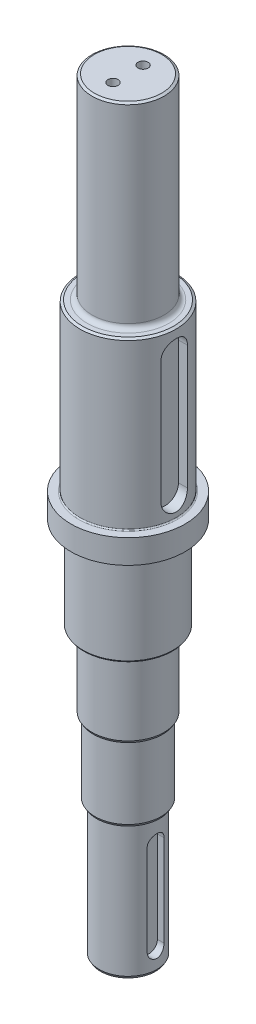
SolidWorks part; units mm, degrees
ref_plane "Front Plane" through (0, 0, 0) normal (0, 0, 1) x (1, 0, 0)
ref_plane "Top Plane" through (0, 0, 0) normal (0, 1, 0) x (1, 0, 0)
ref_plane "Right Plane" through (0, 0, 0) normal (1, 0, 0) x (0, 0, -1)
sketch "Sketch2" plane through (0, 0, 0) normal (0, 0, 1) x (1, 0, 0)
  line L0 (0, -318) -> (0, 318)
  line L1 (0, 318) -> (30, 318)
  line L2 (30, 318) -> (30, 155)
  line L3 (30, 155) -> (40, 155)
  line L4 (40, 155) -> (40, 17)
  line L5 (40, 17) -> (47.5, 17)
  line L6 (47.5, 17) -> (47.5, -3)
  line L7 (47.5, -3) -> (37.5, -3)
  line L8 (37.5, -3) -> (37.5, -80)
  line L9 (37.5, -80) -> (30, -80)
  line L10 (30, -80) -> (30, -144)
  line L11 (30, -144) -> (27.5, -144)
  line L12 (27.5, -144) -> (27.5, -206)
  line L13 (27.5, -206) -> (24, -206)
  line L14 (24, -206) -> (24, -318)
  line L17 (24, -318) -> (0, -318)
  point P4 (0, 0)
  dimension "D1" = 636
  dimension "D2" = 30
  dimension "D3" = 163
  dimension "D4" = 40
  dimension "D5" = 138
  dimension "D6" = 47.5
  dimension "D7" = 20
  dimension "D8" = 37.5
  dimension "D9" = 77
  dimension "D10" = 30
  dimension "D11" = 64
  dimension "D12" = 27.5
  dimension "D13" = 62
  dimension "D14" = 24
revolve "Revolve1" add sketch "Sketch2" angle 360 about L0
chamfer "Chamfer1" distance 2 angle 30 3 edges at (0, -318, -24) (0, 155, -40) (0, 318, -30)
fillet "Fillet1" radius 1 4 edges at (0, -206, -24) (0, -144, -27.5) (0, -80, -30) (0, 17, -40)
fillet "Fillet2" radius 4 1 edges at (0, 155, -30)
fillet "Fillet3" radius 5 1 edges at (0, -3, -37.5)
chamfer "Chamfer2" distance 1 angle 30 1 edges at (0, -80, -37.5)
chamfer "Chamfer3" distance 2 angle 30 1 edges at (0, -206, -27.5)
chamfer "Chamfer4" distance 2 angle 30 1 edges at (0, -144, -30)
sketch "Sketch3" plane through (0, 318, 0) normal (0, 1, 0) x (1, 0, 0)
  line L0 (0, 0) -> (-17.0827, 0) construction
  point P3 (0, 12.5)
  point P4 (0, -12.5)
  dimension "D1" = 25
hole_wizard "M10 Tapped Hole1" positions "Sketch4" profile "Sketch5" tap size "M10" standard "GB"
sketch "Sketch4" plane through (0, 318, 0) normal (0, 1, 0) x (1, 0, 0)
  point P0 (0, 12.5)
  point P3 (0, -12.5)
sketch "Sketch5" plane through (0, 318, -12.5) normal (1, 0, 0) x (0, 0, 1)
  line L0 (0, 0) -> (0, 27.0537)
  line L1 (0, 27.0537) -> (4.25, 24.5)
  line L2 (4.25, 24.5) -> (4.25, 0)
  line L5 (4.25, 0) -> (0, 0)
  line L10 (0, 27.0537) -> (-4.25, 24.5) construction
  line L11 (0, -6.35) -> (0, 107.95) construction
  dimension "螺纹孔钻头直径" = 8.5
  dimension "螺纹孔钻头深度" = 24.5
  dimension "导头角度" = 118
cosmetic thread "Cosmetic thread 1" parameters "D1"=20, "D2"=10
cosmetic thread "Cosmetic thread 2" parameters "D1"=20, "D2"=10
sketch "Sketch6" plane through (0, 0, 0) normal (1, 0, 0) x (0, 0, -1)
  line L0 (0, 136) -> (0, 33) construction
  line L1 (11, 136) -> (11, 33)
  line L2 (-11, 136) -> (-11, 33)
  line L3 (47.5, 17) -> (-47.5, 17) construction
  arc A0 (11, 136) -> (-11, 136) centre (0, 136) ccw
  arc A1 (-11, 33) -> (11, 33) centre (0, 33) ccw
  point P2 (0, 84.5)
  dimension "D1" = 22
  dimension "D2" = 103
  dimension "D3" = 16
extrude "Cut-Extrude1" cut sketch "Sketch6" against normal blind 63 from offset 94
sketch "Sketch8" plane through (0, 0, 0) normal (1, 0, 0) x (0, 0, -1)
  line L0 (0, -301) -> (0, -225) construction
  line L1 (-7, -301) -> (-7, -225)
  line L2 (7, -301) -> (7, -225)
  line L3 (-22.8453, -318) -> (22.8453, -318) construction
  arc A0 (-7, -301) -> (7, -301) centre (0, -301) ccw
  arc A1 (7, -225) -> (-7, -225) centre (0, -225) ccw
  point P2 (0, -263)
  dimension "D1" = 7
  dimension "D2" = 76
  dimension "D3" = 17
extrude "Cut-Extrude2" cut sketch "Sketch8" along normal blind 63 from offset 17.46
